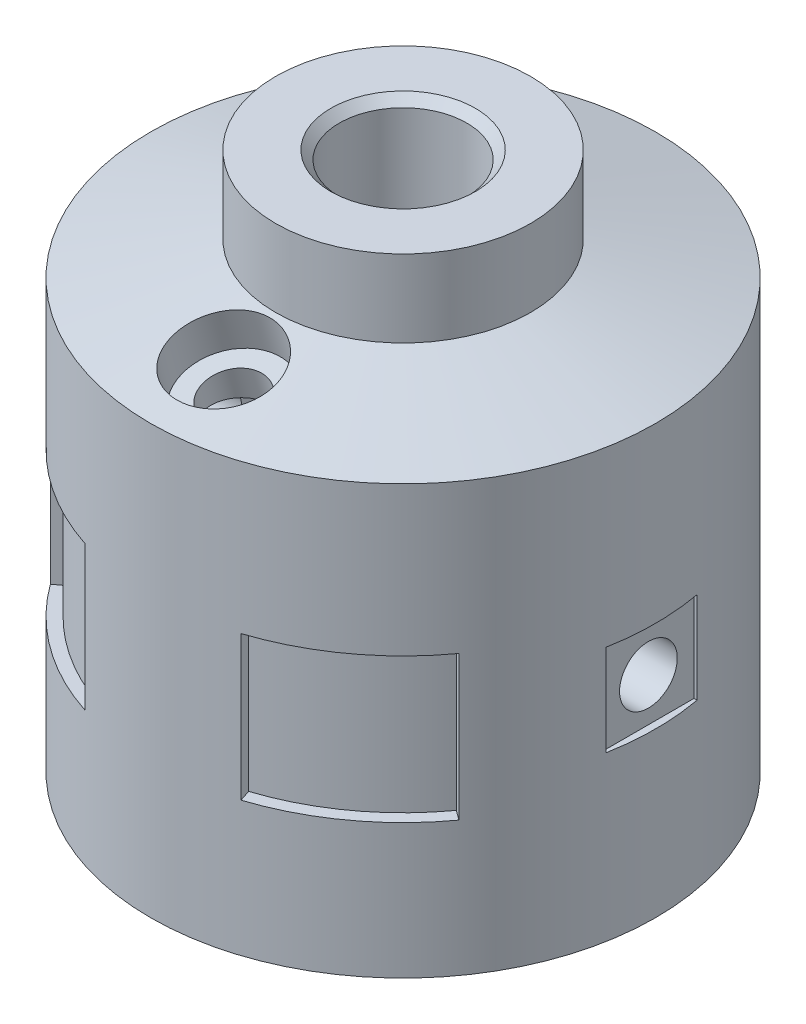
from build123d import *

# Parameters (mm, degrees)
M30_TAPPED_HOLE1_D           = 26.5
M30_TAPPED_HOLE1_DEPTH       = 77.5
M30_TAPPED_HOLE1_CSINK_D     = 30.05
M30_TAPPED_HOLE1_CSINK_ANGLE = 90
M30_TAPPED_HOLE1_TIP         = 7.961403202
SKETCH6_R                    = 40
CUT_EXTRUDE1_DEPTH           = 80
CUT_EXTRUDE2_START           = -43
CUT_EXTRUDE2_DEPTH           = 15
M6_TAPPED_HOLE1_D            = 5
M6_TAPPED_HOLE1_DEPTH        = 12
M6_TAPPED_HOLE1_CSINK_D      = 6.05
M6_TAPPED_HOLE1_CSINK_ANGLE  = 90
M6_TAPPED_HOLE1_TIP          = 1.502151548
CUT_EXTRUDE3_START           = -43.5
SKETCH14_W                   = 3
SKETCH14_H                   = 19
CUT_EXTRUDE3_DEPTH           = 9.5
CUT_EXTRUDE4_DEPTH           = 162.283911163
CUT_EXTRUDE4_DEPTH_BACK      = 162.283911163
SKETCH15_R                   = 6
CUT_EXTRUDE5_DEPTH           = 135.374476743
CUT_EXTRUDE5_DEPTH_BACK      = 10


with BuildPart() as part:
    # Sketch2 → Revolve1 (revolve)
    with BuildSketch(Plane.XY, mode=Mode.PRIVATE) as revolve1_sk:
        Polygon((0, 0), (0, 112), (-26.5, 112), (-26.5, 95.966679003), (-52.5, 89), (-52.5, 0), align=None)
    revolve(revolve1_sk.sketch.rotate(Axis((0, 102.234109067, 0), (0, -1, 0)), 270), axis=Axis((0, 102.234109067, 0), (0, -1, 0)))

    # M30 Tapped Hole1
    with Locations(Plane(origin=(0, 112, 0), x_dir=(1, 0, 0), z_dir=(0, 1, 0))):
        with Locations((0, 0)):
            CounterSinkHole(M30_TAPPED_HOLE1_D / 2, M30_TAPPED_HOLE1_CSINK_D / 2, depth=M30_TAPPED_HOLE1_DEPTH, counter_sink_angle=M30_TAPPED_HOLE1_CSINK_ANGLE)
            with Locations((0, 0, -(M30_TAPPED_HOLE1_DEPTH + M30_TAPPED_HOLE1_TIP / 2))):  # 118° drill point
                Cone(0, M30_TAPPED_HOLE1_D / 2, M30_TAPPED_HOLE1_TIP, mode=Mode.SUBTRACT)

    # Sketch6 → Cut-Extrude1 (cut)
    with BuildSketch(Plane.XZ):
        with Locations(Location((0, 0, 0), (0, 0, 270))):
            Circle(SKETCH6_R)
    extrude(amount=-CUT_EXTRUDE1_DEPTH, mode=Mode.SUBTRACT)

    # Sketch8 → Cut-Extrude2 (cut, symmetric)
    with BuildSketch(Plane.XZ.offset(CUT_EXTRUDE2_START)):
        with BuildLine():
            Line((-15.450849719, 47.552825815), (-16.223392205, 49.930467105))
            ThreePointArc((-16.223392205, 49.930467105), (-30.858725745, 42.473392205), (-42.473392205, 30.858725745))
            Line((-42.473392205, 30.858725745), (-40.450849719, 29.389262615))
            ThreePointArc((-40.450849719, 29.389262615), (-29.389262615, 40.450849719), (-15.450849719, 47.552825815))
        make_face()
    cut_extrude2 = extrude(amount=CUT_EXTRUDE2_DEPTH, both=True, mode=Mode.SUBTRACT)

    # Mirror1: Cut-Extrude2 across plane
    add(cut_extrude2.mirror(Plane(origin=(0, 0, 0), x_dir=(0, 0, 1), z_dir=(1, 0, 0))), mode=Mode.SUBTRACT)

    # M6 Tapped Hole1
    with Locations(Plane.XZ):
        with Locations((-45, 0), (45, 0)):
            CounterSinkHole(M6_TAPPED_HOLE1_D / 2, M6_TAPPED_HOLE1_CSINK_D / 2, depth=M6_TAPPED_HOLE1_DEPTH, counter_sink_angle=M6_TAPPED_HOLE1_CSINK_ANGLE)
            with Locations((0, 0, -(M6_TAPPED_HOLE1_DEPTH + M6_TAPPED_HOLE1_TIP / 2))):  # 118° drill point
                Cone(0, M6_TAPPED_HOLE1_D / 2, M6_TAPPED_HOLE1_TIP, mode=Mode.SUBTRACT)

    # Sketch14 → Cut-Extrude3 (cut, symmetric)
    with BuildSketch(Plane.XZ.offset(CUT_EXTRUDE3_START)):
        with Locations((52.5, 0)):
            Rectangle(SKETCH14_W, SKETCH14_H)
        with Locations((-52.5, 0)):
            Rectangle(SKETCH14_W, SKETCH14_H)
    extrude(amount=CUT_EXTRUDE3_DEPTH, both=True, mode=Mode.SUBTRACT)

    # Sketch15 → Cut-Extrude4 (cut, two sides: drawn at the far end of the back side and taken through both)
    with BuildSketch(Plane.ZY.offset(51).offset(-CUT_EXTRUDE4_DEPTH_BACK)):
        with Locations((0, 43)):
            Circle(SKETCH15_R)
    extrude(amount=CUT_EXTRUDE4_DEPTH + CUT_EXTRUDE4_DEPTH_BACK, mode=Mode.SUBTRACT)

    # Sketch16 → Cut-Extrude5 (cut, two sides: drawn at the far end of the back side and taken through both)
    with BuildSketch(Plane.XZ.offset(-CUT_EXTRUDE5_DEPTH_BACK)):
        with BuildLine():
            Line((10.607312288, 42), (-10.607312288, 42))
            ThreePointArc((-10.607312288, 42), (-19.596893761, 39.007806833), (-25, 31.224989992))
            ThreePointArc((-25, 31.224989992), (0, 40), (25, 31.224989992))
            ThreePointArc((25, 31.224989992), (19.596893761, 39.007806833), (10.607312288, 42))
        make_face()
        with BuildLine():
            Line((10.607312288, -42), (-10.607312288, -42))
            ThreePointArc((-10.607312288, -42), (-19.596893761, -39.007806833), (-25, -31.224989992))
            ThreePointArc((-25, -31.224989992), (0, -40), (25, -31.224989992))
            ThreePointArc((25, -31.224989992), (19.596893761, -39.007806833), (10.607312288, -42))
        make_face()
    extrude(amount=CUT_EXTRUDE5_DEPTH + CUT_EXTRUDE5_DEPTH_BACK, mode=Mode.SUBTRACT)

    # Sketch17 → Cut-Revolve4 (revolve, cut)
    with BuildSketch(Plane(origin=(0, 0, 0), x_dir=(0, 0, -1), z_dir=(1, 0, 0))):
        Polygon((-37.77510745, 94.609566001), (-47.434365712, 92.02137555), (-44.846175261, 82.362117287), (-40.982471956, 83.397393467), (-38.749196282, 75.062695183), (-32.953641324, 76.615609453), align=None)
    revolve(axis=Axis((0, 99.934460592, 39.201908655), (0, -0.96592582628907, -0.2588190451025148)), mode=Mode.SUBTRACT)


solid = part.part
